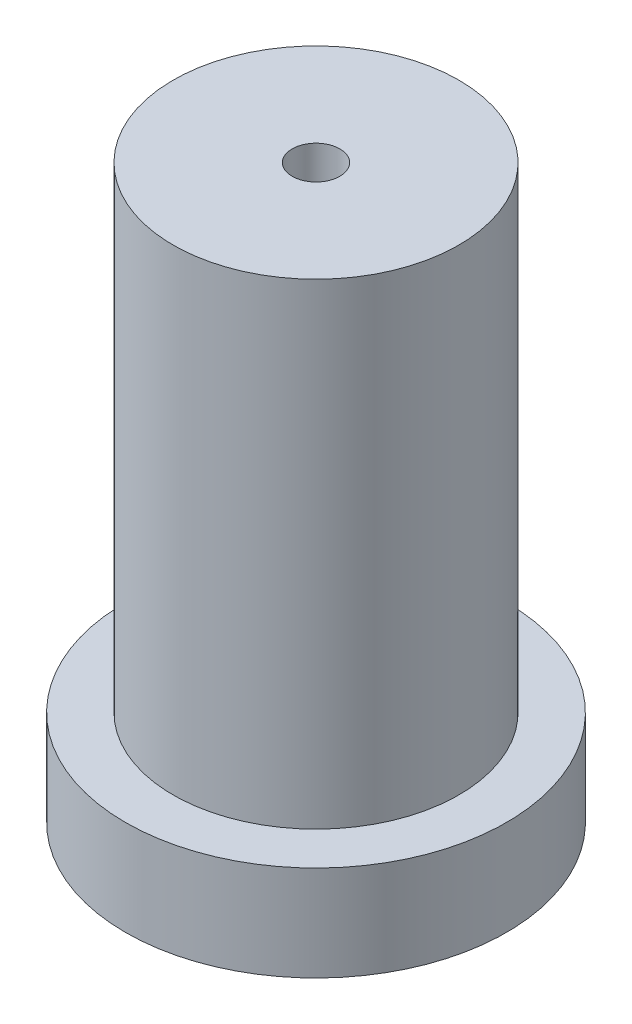
from build123d import *


with BuildPart() as part:
    # 草图1 → 旋转1 (revolve)
    with BuildSketch(Plane.XY, mode=Mode.PRIVATE) as revolve_1_sk:
        Polygon((0.25, 3.773087071), (0.25, -2.226912929), (2, -2.226912929), (2, -1.226912929), (1.5, -1.226912929), (1.5, 3.773087071), align=None)
    revolve(revolve_1_sk.sketch.rotate(Axis((0, 0, 0), (0, 1, 0)), 90), axis=Axis((0, 0, 0), (0, 1, 0)))


solid = part.part
